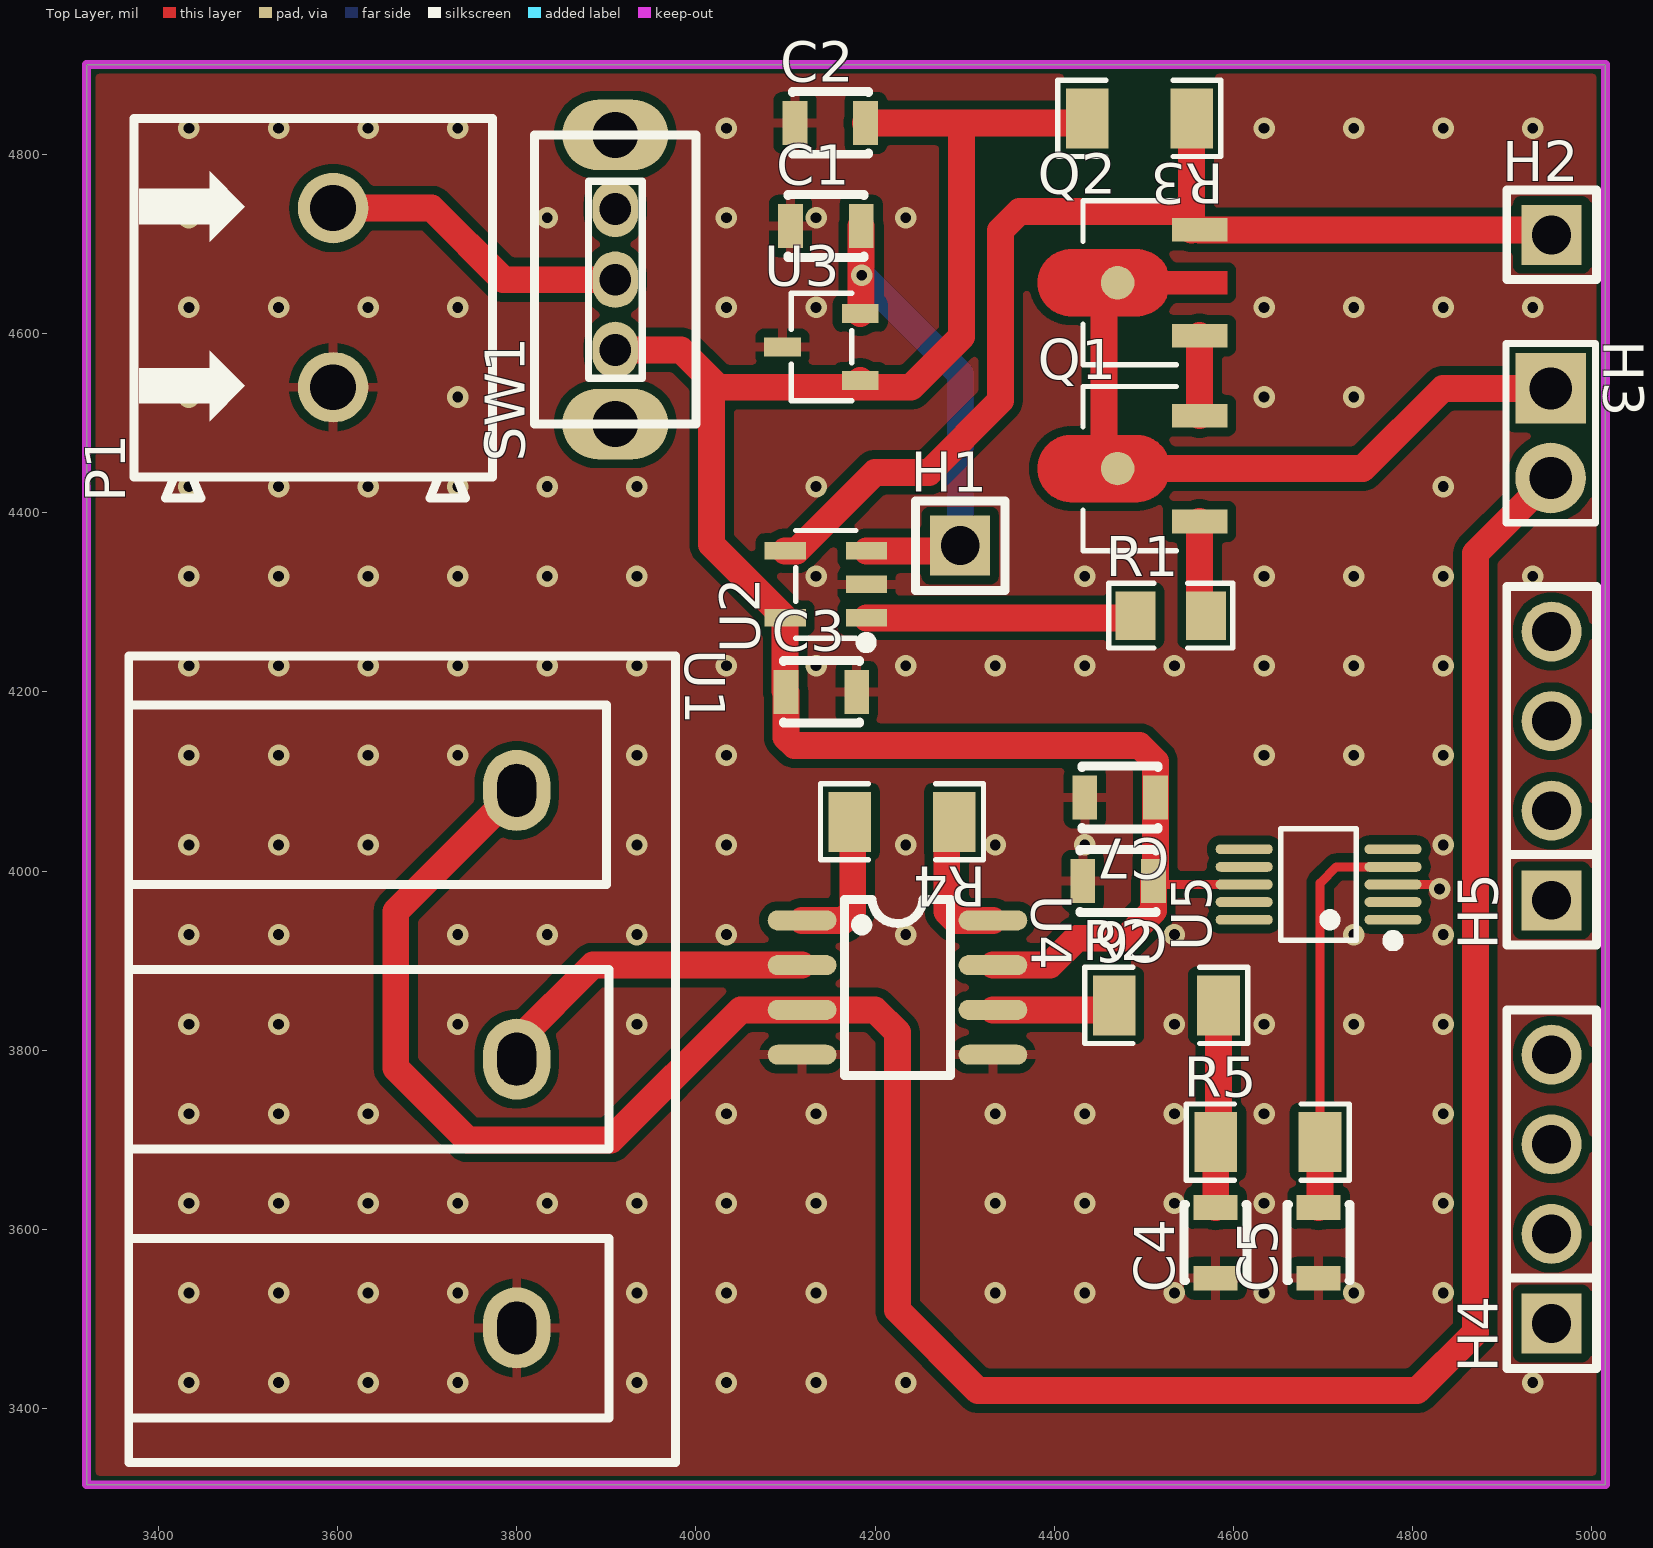
[diagram p0: Top Layer view]
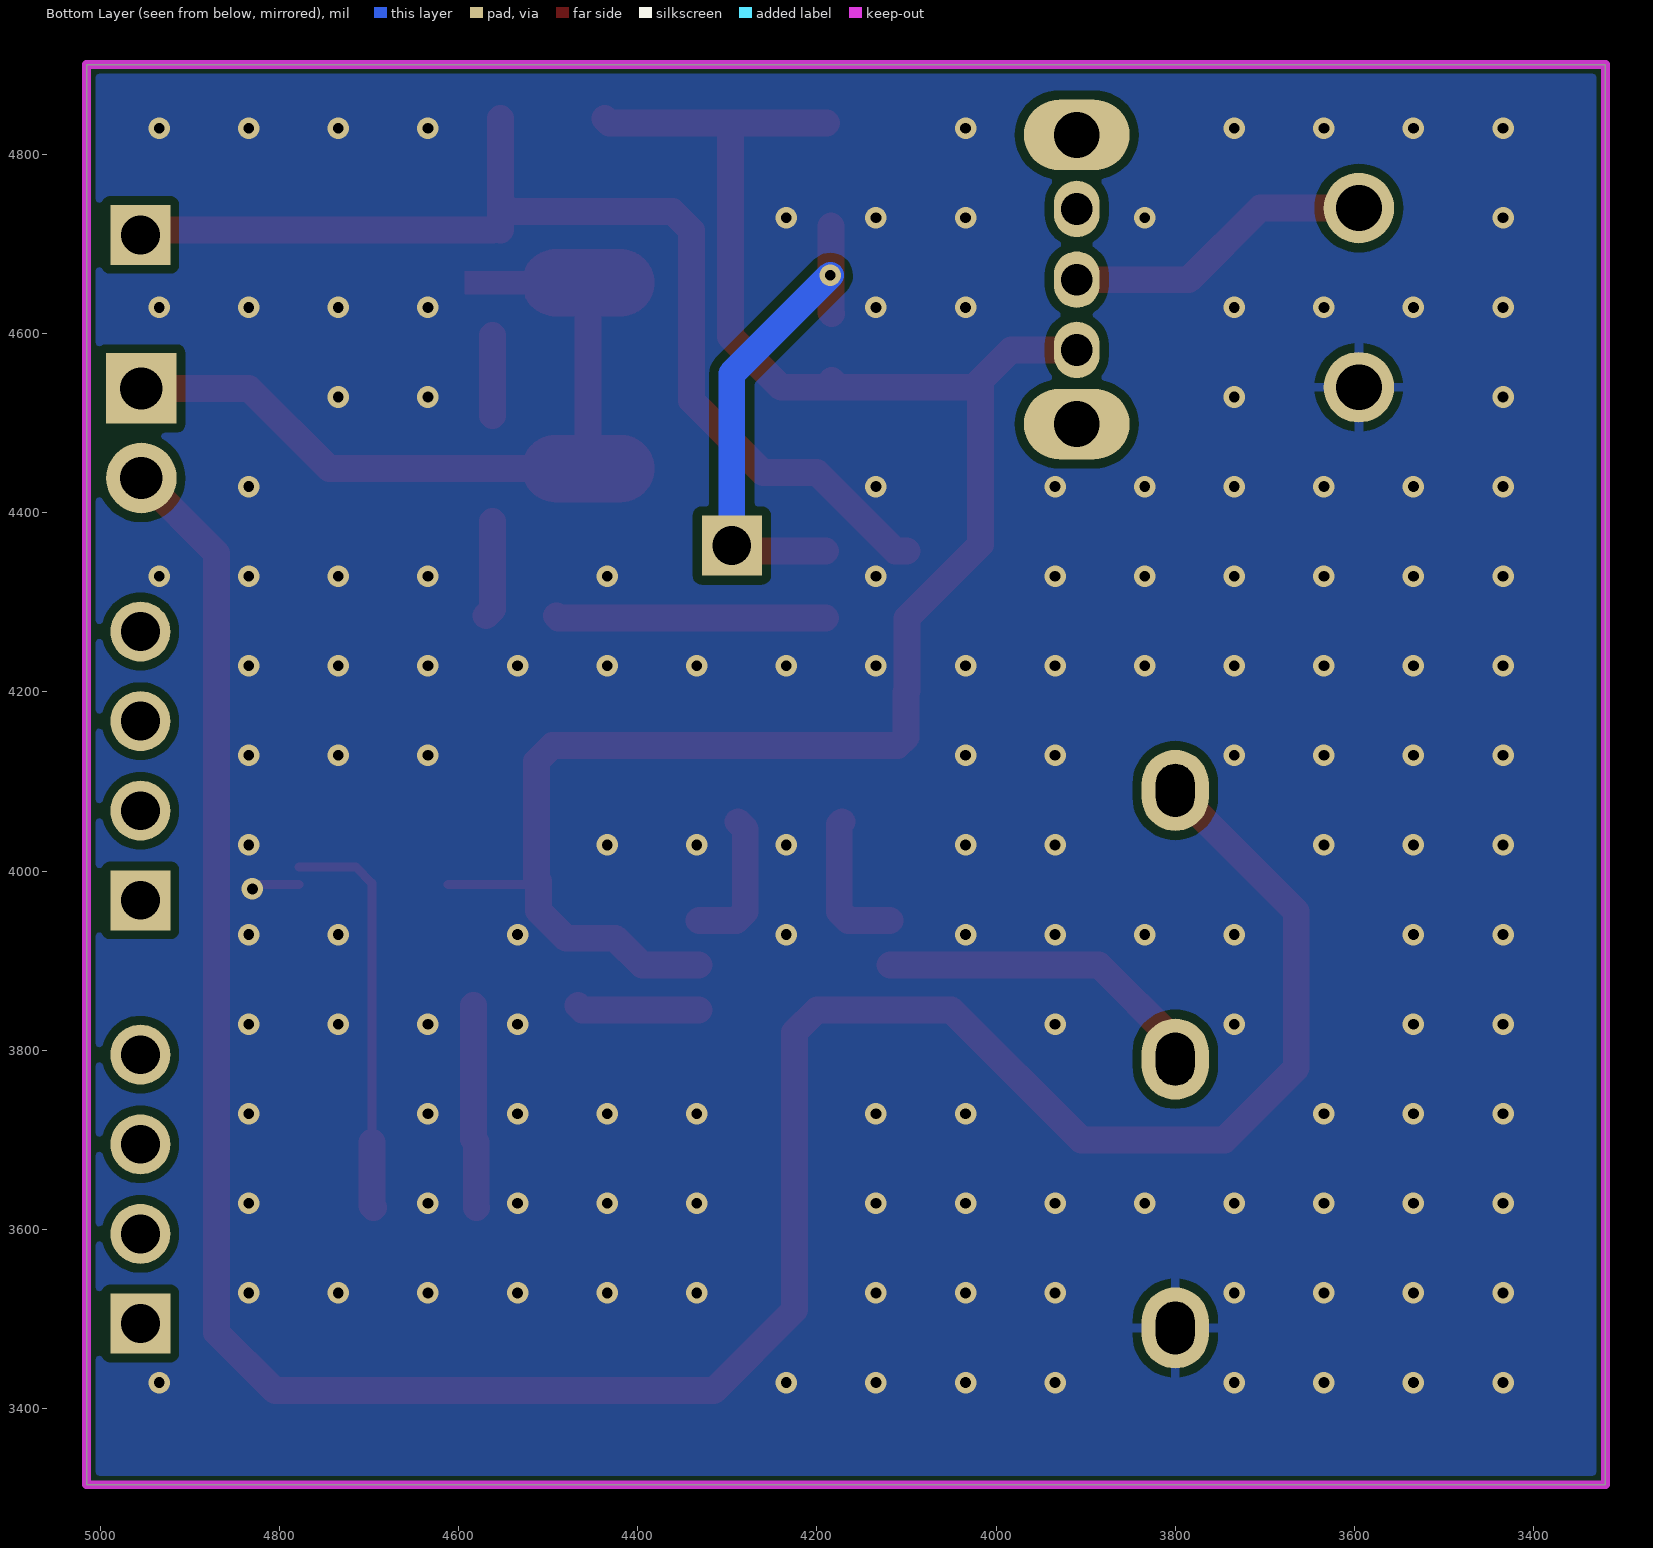
[diagram p1: Bottom Layer view, seen from below]
# Altium PCB MISC52115.pcbdoc
Units mil, origin at the board's own origin, x right, y up, seen from the top; angles counter-clockwise.
Board outline 1695 x 1585 mil, 2 copper layers (Top Layer, Bottom Layer), stack 62.206 mil thick; 26 components, 24 nets, 78 pads, 146 vias.

## Layer stack, top to bottom
Top Solder Mask Layer: solder mask 0.394, Dk 3.3
Top Layer: signal copper 1.379
Dielectric1: surface 59.449, FR4, Dk 4.5
Bottom Layer: signal copper 1.378
Bottom Solder Mask Layer: solder mask 0.394, Dk 3.3

## Board outline
3320,4900 3320,3315 5015,3315 5015,4900

## Design rules (kind name [scope] priority, off if disabled: settings)
BoardOutlineClearance copperThickness2oz_1 [All] p2 off: genericclearance=7.99 ignorepadtopadclearanceinfootprint=FALSE except(0: Arc-SplitContinuation Track-SplitContinuation SMDPad-SplitContinuation THPad-SplitContinuation Via-SplitContinuation Fill-SplitContinuation Region-SplitContinuation Poly-SplitContinuation Text-SplitContinuation Hole-SplitContinuation; 5.98: Arc-CutoutEdge SMDPad-CutoutEdge THPad-CutoutEdge Via-CutoutEdge Fill-CutoutEdge Region-CutoutEdge Text-CutoutEdge; 6.93: Hole-OutlineEdge Hole-CutoutEdge; 10: Poly-OutlineEdge Poly-CutoutEdge; 11.81: Arc-OutlineEdge Track-OutlineEdge SMDPad-OutlineEdge THPad-OutlineEdge Via-OutlineEdge Fill-OutlineEdge Region-OutlineEdge Text-OutlineEdge Track-CutoutEdge)
BoardOutlineClearance copperThickness1oz_1 [All] p4: genericclearance=4.02 ignorepadtopadclearanceinfootprint=FALSE except(0: Arc-SplitContinuation Track-SplitContinuation SMDPad-SplitContinuation THPad-SplitContinuation Via-SplitContinuation Fill-SplitContinuation Region-SplitContinuation Poly-SplitContinuation Text-SplitContinuation Hole-SplitContinuation; 6: SMDPad-CutoutEdge THPad-CutoutEdge Via-CutoutEdge Fill-CutoutEdge Region-CutoutEdge Text-CutoutEdge; 6.93: Hole-OutlineEdge Hole-CutoutEdge; 10: Poly-OutlineEdge Poly-CutoutEdge; 11.8: Arc-OutlineEdge Track-OutlineEdge SMDPad-OutlineEdge THPad-OutlineEdge Via-OutlineEdge Fill-OutlineEdge Region-OutlineEdge Text-OutlineEdge; 11.81: Arc-CutoutEdge Track-CutoutEdge)
Clearance copperThickness2oz [All] p1 off: gap=7.99 ignorepadtopadclearanceinfootprint=FALSE except(5.98: SMDPad-Track SMDPad-SMDPad THPad-Track SMDPad-THPad THPad-THPad Track-Via SMDPad-Via THPad-Via Via-Via Fill-Track Region-Track Fill-SMDPad Region-SMDPad Fill-THPad Region-THPad Fill-Via Region-Via Fill-Fill Fill-Region Region-Region Arc-Track Arc-SMDPad Arc-THPad Arc-Via Fill-Arc Region-Arc Arc-Arc Text-Track SMDPad-Text Text-THPad Text-Via Fill-Text Region-Text Arc-Text Text-Text; 6.93: Hole-Track Hole-SMDPad Hole-THPad Hole-Via Fill-Hole Region-Hole Hole-Arc Hole-Text; 10: Poly-Track Poly-SMDPad Poly-THPad Poly-Via Poly-Fill Poly-Region Poly-Poly Poly-Arc Poly-Text Poly-Hole)
Clearance copperThickness1oz [All] p3: gap=4.02 ignorepadtopadclearanceinfootprint=FALSE except(5.98: SMDPad-Track SMDPad-SMDPad THPad-Track SMDPad-THPad THPad-THPad Track-Via SMDPad-Via THPad-Via Via-Via Fill-Track Region-Track Fill-SMDPad Region-SMDPad Fill-THPad Region-THPad Fill-Via Region-Via Fill-Fill Fill-Region Region-Region; 6: Arc-Track Arc-SMDPad Arc-THPad Arc-Via Fill-Arc Region-Arc Arc-Arc Text-Track SMDPad-Text Text-THPad Text-Via Fill-Text Region-Text Arc-Text Text-Text; 6.93: Hole-Track Hole-SMDPad Hole-THPad Hole-Via Fill-Hole Region-Hole Hole-Arc Hole-Text; 10: Poly-Track Poly-SMDPad Poly-THPad Poly-Via Poly-Fill Poly-Region Poly-Poly Poly-Arc Poly-Text Poly-Hole)
DiffPairsRouting differentialPair [All] p1: maxlimit=6 minlimit=6 mostfreqgap=6 toplayer_minwidth=5 toplayer_prefwidth=10 toplayer_maxwidth=100 toplayer_mingap=6 toplayer_prefgap=6 toplayer_maxgap=6 bottomlayer_minwidth=5 bottomlayer_prefwidth=10 bottomlayer_maxwidth=100 bottomlayer_mingap=6 bottomlayer_prefgap=6 bottomlayer_maxgap=6 maxuncoupledlength=10
HoleToHoleClearance otherClearance [All] p1: gap=11.81 allowstackedmicrovias=TRUE
Length netLength [All] p1: minlimit=0 maxlimit=0
MatchedLengths netLengthTolerance [All] p1: tolerance=1000
PasteMaskExpansion pasteMaskExpansion [All] p1: expansion=0
PlaneConnect innerPlane [All] p1: planeconnectstyle=Relief reliefexpansion=20 reliefentries=4 reliefconductorwidth=10 reliefairgap=10
PolygonConnect copperRegion [(InNet('GND'))] p1: connectstyle=Relief reliefconductorwidth=10 reliefentries=4 polygonreliefangle="90 Angle" airgapwidth=10 via.connectstyle=Relief via.reliefconductorwidth=10 via.reliefentries=4 via.polygonreliefangle="90 Angle" via.airgapwidth=10
RoutingVias viaSize [All] p1: holewidth=12.01 width=24.02 viastyle="Through Hole" minholewidth=11.81 minwidth=19.68 maxholewidth=248.03 maxwidth=393.7
SolderMaskExpansion solderMaskExpansion [IsVia] p1: expansion=-1000 istentingtop=TRUE
SolderMaskExpansion solderMaskExpansion [All] p2: expansion=2 istentingtop=FALSE
Width copperThickness2oz_2 [All] p1 off: maxlimit=100 minlimit=8 preferedwidth=10
Width copperThickness1oz_2 [All] p2: maxlimit=100 minlimit=5 preferedwidth=10

## Components (designator, comment, footprint, x,y, rotation, side; value= is the part's Value field where it differs from the comment)
C1 "100nF" CAP-SMD_L2.0-W1.25 4145,4720 r0 top
C2 "100nF" CAP-SMD_L2.0-W1.25 4150,4835 r0 top
C3 "100nF" CAP-SMD_L2.0-W1.25 4140,4200 r0 top
C4 "1uF" CAP-SMD_L2.0-W1.25 4580,3585 r90 top
C5 "4.7nf" CAP-SMD_L2.0-W1.25 4695,3585 r90 top
C6 "100nf" CAP-SMD_L2.0-W1.25 4471.28,3988.83 r180 top
C7 "100nf" CAP-SMD_L2.0-W1.25 4473.49,4082.08 r180 top
H1 "PZ254V-11-01P" HDR-TH_1P-P2.54-V-M 4294.96,4363.25 r0 top
H2 "PZ254V-11-01P" HDR-TH_1P-P2.54-V-M 4955,4710 r0 top
H3 "PZ254V-11-02P" HDR-TH_2P-P2.54-V-M 4954,4488.67 r270 top
H4 "PZ254V-11-04P" HDR-TH_4P-P2.54-V-M 4955,3645 r90 top
H5 "PZ254V-11-04P" HDR-TH_4P-P2.54-V-M 4955,4117.33 r90 top
P1 "WJ500V-5.08-2P" CONN-TH_2P-P5.00_WJ500V-5.08-2P 3595,4640 r90 top
Q1 "2SA1201" SOT-89-3_L4.5-W2.5-P1.50-LS4.2-BR 4508.73,4449.26 r0 top
Q2 "2SA1201" SOT-89-3_L4.5-W2.5-P1.50-LS4.2-BR 4508.73,4656.61 r0 top
R1 "10kΩ" R0805 4530,4285 r0 top
R2 "1KΩ" R1206 4525,3850 r0 top
R3 "2.7KΩ" R1206 4495,4840 r180 top
R4 "6KΩ" R1206 4230,4055 r180 top
R5 "1KΩ" R1206 4638.39,3697.51 r0 top
SW1 "" 拨动开关 3910,4655 r90 top
U1 "JL762-76203BA1" CONN-TH_JL762-76203BA1 3800,3790 r270 top
U2 "SGM8551XN5G/TR" SOT-23-5_L3.0-W1.7-P0.95-LS2.8-BL 4145,4320 r90 top
U3 "REF3025AIDBZT" SOT-23-3_L3.0-W1.7-P0.95-LS2.9-BR 4140,4585 r0 top
U4 "AD623ARZ-R7" SOIC-8_L5.0-W4.0-P1.27-LS6.0-BL 4225,3870 r270 top
U5 "GD30AD3344" MSOP-10_L3.0-W3.0-P0.50-LS5.0-BL 4695,3985 r90 top

## Footprints (in the part's own frame and the unit in brackets; to place one, negate y for a bottom-side part, rotate by r counter-clockwise, add the part's x,y. Pads: shape width x height; smd on the part's side, far side on the other; paste and mask are expansions set on the pad)
CAP-SMD_L2.0-W1.25 [mm]
  rect 0.7x1.25 smd: 1(-1,0) 2(1,0)
  silkscreen extent -1.08,-0.89 1.08,0.89
CONN-TH_2P-P5.00_WJ500V-5.08-2P [mm]
  round 2 hole 1.3: 1(-2.54,0) 2(2.54,0)
  silkscreen extent -5.68,-4.52 5.08,5.64
CONN-TH_JL762-76203BA1 [mm]
  oval 2.3x1.9 hole 1.1 slot 1.5 at 0 deg: 1(-7.62,0) 2(0,0) 3(7.62,0)
  silkscreen extent -11.43,-11 11.43,4.5
HDR-TH_1P-P2.54-V-M [mm]
  rect 1.7x1.7 hole 1.1: 1(0,0)
  silkscreen extent -1.27,-1.27 1.27,1.27
HDR-TH_2P-P2.54-V-M [mm]
  rect 2x2 hole 1.2: 1(-1.27,0)
  round 2 hole 1.2: 2(1.27,0)
  silkscreen extent -2.54,-1.27 2.54,1.27
HDR-TH_4P-P2.54-V-M [mm]
  rect 1.7x1.7 hole 1.1: 1(-3.81,0)
  round 1.7 hole 1.1: 2(-1.27,0) 3(1.27,0) 4(3.81,0)
  silkscreen extent -5.08,-1.27 5.08,1.27
MSOP-10_L3.0-W3.0-P0.50-LS5.0-BL [mm]
  oval 0.28x1.62 smd: 1(-1,-2.11) 2(-0.5,-2.11) 3(0,-2.11) 4(0.5,-2.11) 5(1,-2.11) 6(1,2.11) 7(0.5,2.11) 8(0,2.11) 9(-0.5,2.11) 10(-1,2.11)
  silkscreen extent -1.74,-2.26 1.58,1.07
R0805 [mm]
  rect 1.133x1.377 smd paste-100 mask+0.051: 1(-1,0) 2(1,0)
  silkscreen extent -1.76,-0.92 1.76,0.92
R1206 [mil]
  rect 47.54x66.97 smd paste-3937.01 mask+2: 1(-58.22,0) 2(58.22,0)
  silkscreen extent -91,-42 91,42
SOIC-8_L5.0-W4.0-P1.27-LS6.0-BL [mil]
  oval 22.38x76.78 smd: 1(-75,-106.5) 2(-25,-106.5) 3(25,-106.5) 4(75,-106.5) 5(75,106.5) 6(25,106.5) 7(-25,106.5) 8(-75,106.5)
  silkscreen extent -98,-59 98,59
SOT-23-3_L3.0-W1.7-P0.95-LS2.9-BR [mil]
  rect 40.85x20.95 smd: 1(43.36,-37.4) 2(43.36,37.4) 3(-43.36,0)
  silkscreen extent -34,-60 34,60
SOT-23-5_L3.0-W1.7-P0.95-LS2.8-BL [mm]
  rect 0.49x1.157 smd: 1(-0.95,-1.154) 2(0,-1.154) 3(0.95,-1.154)
  rect 0.49x1.175 smd: 4(0.95,1.154) 5(-0.95,1.154)
  silkscreen extent -1.8,-1.29 1.53,0.85
SOT-89-3_L4.5-W2.5-P1.50-LS4.2-BR [mm]
  rect 1.575x0.672 smd: 1(1.356,-1.5) 3(1.356,1.5)
  round 0.95 smd: 2(-0.966,0)
  Top Layer region: -2.283,0.95 -0.429,0.95 -0.384,0.949 -0.34,0.946 -0.296,0.94 -0.252,0.933 -0.208,0.924 -0.165,0.912 -0.123,0.899 -0.081,0.884 -0.04,0.866 0,0.847 0.04,0.826 0.078,0.803 0.115,0.779 0.151,0.752 0.185,0.724 0.219,0.695 0.251,0.664 0.281,0.631 0.31,0.597 0.337,0.562 0.362,0.525 0.386,0.488 0.408,0.449 0.428,0.409 0.447,0.33 2.144,0.33 2.144,-0.33 0.447,-0.33 0.428,-0.409 0.408,-0.449 0.386,-0.488 0.362,-0.526 0.337,-0.562 0.31,-0.597 0.281,-0.631 0.251,-0.664 0.219,-0.695 0.185,-0.725 0.151,-0.753 0.115,-0.779 0.078,-0.804 0.04,-0.827 0,-0.848 -0.04,-0.867 -0.081,-0.884 -0.123,-0.899 -0.165,-0.913 -0.208,-0.924 -0.252,-0.934 -0.296,-0.941 -0.34,-0.946 -0.384,-0.949 -0.429,-0.95 -2.283,-0.95 -2.328,-0.949 -2.372,-0.946 -2.416,-0.941 -2.46,-0.934 -2.504,-0.924 -2.547,-0.913 -2.589,-0.899 -2.631,-0.884 -2.672,-0.867 -2.713,-0.848 -2.752,-0.827 -2.79,-0.804 -2.827,-0.779 -2.863,-0.753 -2.898,-0.725 -2.931,-0.695 -2.963,-0.664 -2.993,-0.631 -3.022,-0.597 -3.049,-0.562 -3.075,-0.526 -3.098,-0.488 -3.12,-0.449 -3.141,-0.409 -3.159,-0.369 -3.175,-0.327 -3.189,-0.285 -3.202,-0.242 -3.212,-0.199 -3.22,-0.155 -3.227,-0.111 -3.231,-0.067 -3.233,-0.022 -3.233,0.022 -3.231,0.067 -3.227,0.111 -3.22,0.155 -3.212,0.199 -3.202,0.242 -3.189,0.285 -3.175,0.327 -3.159,0.369 -3.141,0.409 -3.12,0.449 -3.098,0.488 -3.075,0.525 -3.049,0.562 -3.022,0.597 -2.993,0.631 -2.963,0.664 -2.931,0.695 -2.898,0.724 -2.863,0.752 -2.827,0.779 -2.79,0.803 -2.752,0.826 -2.713,0.847 -2.672,0.866 -2.631,0.884 -2.589,0.899 -2.547,0.912 -2.504,0.924 -2.46,0.933 -2.416,0.94 -2.372,0.946 -2.328,0.949
  silkscreen extent -1.95,-2.33 0.7,2.33
拨动开关 [mil]
  oval 63x51.2 hole 35.4 paste+0 mask+2: 1(-73.4,0) 2(5,0) 3(84,0)
  oval 78.7x118.1 hole 51.2 paste+0 mask+2: 4(166.7,0) 5(-156.1,0)
  silkscreen extent -156,-90 167,90

## Via types
v1: diameter 24.02, hole 12, Top Layer to Bottom Layer, 146 vias

## Nets (pads, with @x,y where several pads share a name; then routed paths per layer and width w, separated by ;. In a path a pad name is that pad's centre, name@x,y a point inside that pad or via, vN(x,y) a via of type N, cw(c..) or ccw(c..) an arc to the next point about the centre after c; other vN are vias at no path point)
$1N4: C1.2 H1.1 U2.3 U3.2 | length 552.3
  Top Layer w30: U3.2 4184.37,4623.41 C1.2 ; U2.3 4289.11,4357.4 H1.1
  Bottom Layer w30: v1(4185,4665) 4294.96,4555.04 H1.1
$1N8: R1.1 U2.1 | length 301.2
  Top Layer w30: U2.1 4488.23,4282.6 R1.1
$1N10: Q1.1 R1.2 | length 108.2
  Top Layer w30: Q1.1 4562.13,4292.24 R1.2
$1N11: Q1.3 Q2.1 | length 89.2
  Top Layer w30: Q1.3 Q2.1
$1N12: H2.1 Q2.3 R3.1 U2.4 | length 1245.8
  Top Layer w30: U2.4 4112.4,4357.4 4200,4445 4260,4445 4340,4525 4340,4715 4361.21,4736.21 4542.56,4736.21 4553.22,4746.87 ; Q2.3@4553.22,4715.67 4553.22,4746.87 ; R3.1 4553.22,4746.87 ; Q2.3 4949.33,4715.67 H2.1
$1N18: H3.1 Q1.2 Q2.2 | length 743.1
  Top Layer w30: Q2.2@4455.34,4656.61 4455.34,4449.25 4744.25,4449.25 4833.67,4538.67 H3.1
$1N34: R4.2 U4.1 | length 162
  Top Layer w30: U4.1 4165,3945 4175,3955 4175,4051.78 R4.2
$1N35: U1.2 U4.2 | length 373.7
  Top Layer w30: U1.2 3800,3810 3885,3895 U4.2
$1N36: R4.1 U4.8 | length 159
  Top Layer w30: R4.1 4280,4046.78 4280,3955 4290,3945 U4.8
$1N40: R2.1 U4.6 | length 137.4
  Top Layer w30: U4.6 4461.78,3845 R2.1
$1N41: C4.2 R2.2 R5.1 | length 227
  Top Layer w30: C4.2 4580.17,3624.54 R5.1 4583.22,3700.57 R2.2
$1N43: C5.2 R5.2 U5.4 | length 451.9
  Top Layer w10: R5.2 4696.61,3986.61 4714.69,4004.69 U5.4
  Top Layer w30: C5.2 4696.61,3625.98 R5.2
$1N48: H4.1
$1N49: H4.2
$1N50: H4.3
$1N51: H4.4
$1N52: H5.1
$1N53: H5.2
$1N54: H5.3
$1N55: H5.4
$1N62: P1.2 SW1.2 | length 348.1
  Top Layer w30: P1.2 3705,4740 3785,4660 SW1.2
+5V: C2.2 C3.1 C6.1 C7.1 R3.2 SW1.1 U2.5 U3.1 U4.7 U5.8 | length 2256.4
  Top Layer w10: C6.1 4514.48,3985 U5.8
  Top Layer w30: SW1.1 3983.4,4581.6 4017.56,4547.44 ; U3.1 U3.1@4175.76,4540 ; C2.2 4296.39,4835 ; U4.7 4395,3895 4425,3925 4480,3925 4510.65,3955.65 C6.1 4512.86,3991.04 C7.1 4512.86,4122.14 4495,4140 4110,4140 4100.63,4149.37 C3.1 4099.58,4201.05 U2.5 4017.56,4364.62 4017.56,4547.44 ; R3.2 4431.78,4835 4296.39,4835 ; 4017.56,4547.44 4025,4540 U3.1@4175.76,4540 ; U3.1@4175.76,4540 4240,4540 4296.39,4596.39 4296.39,4835
GND: C1.1 C2.1 C3.2 C4.1 C5.1 C6.2 C7.2 P1.1 U1.3 U2.2 U3.3 U4.4 U4.5 U5.3 | length 54
  Top Layer w10: U5.3 4825,3985 v1(4830,3980)
  other v1: 3434.1,3429.1 3534.1,3429.1 3634.1,3429.1 3734.1,3429.1 3934.1,3429.1 4034.1,3429.1 4134.1,3429.1 4234.1,3429.1 4934.1,3429.1 3434.1,3529.1 3534.1,3529.1 3634.1,3529.1 3734.1,3529.1 3934.1,3529.1 4034.1,3529.1 4134.1,3529.1 4334.1,3529.1 4434.1,3529.1 4534.1,3529.1 4634.1,3529.1 4734.1,3529.1 4834.1,3529.1 3434.1,3629.1 3534.1,3629.1 3634.1,3629.1 3734.1,3629.1 3834.1,3629.1 3934.1,3629.1 4034.1,3629.1 4134.1,3629.1 4334.1,3629.1 4434.1,3629.1 4534.1,3629.1 4634.1,3629.1 4834.1,3629.1 3434.1,3729.1 3534.1,3729.1 3634.1,3729.1 4034.1,3729.1 4134.1,3729.1 4334.1,3729.1 4434.1,3729.1 4534.1,3729.1 4634.1,3729.1 4834.1,3729.1 3434.1,3829.1 3534.1,3829.1 3734.1,3829.1 3934.1,3829.1 4534.1,3829.1 4634.1,3829.1 4734.1,3829.1 4834.1,3829.1 3434.1,3929.1 3534.1,3929.1 3734.1,3929.1 3834.1,3929.1 3934.1,3929.1 4034.1,3929.1 4234.1,3929.1 4534.1,3929.1 4734.1,3929.1 4834.1,3929.1 3434.1,4029.1 3534.1,4029.1 3634.1,4029.1 3934.1,4029.1 4034.1,4029.1 4234.1,4029.1 4334.1,4029.1 4434.1,4029.1 4834.1,4029.1 3434.1,4129.1 3534.1,4129.1 3634.1,4129.1 3734.1,4129.1 3934.1,4129.1 4034.1,4129.1 4634.1,4129.1 4734.1,4129.1 4834.1,4129.1 3434.1,4229.1 3534.1,4229.1 3634.1,4229.1 3734.1,4229.1 3834.1,4229.1 3934.1,4229.1 4034.1,4229.1 4134.1,4229.1 4234.1,4229.1 4334.1,4229.1 4434.1,4229.1 4534.1,4229.1 4634.1,4229.1 4734.1,4229.1 4834.1,4229.1 3434.1,4329.1 3534.1,4329.1 3634.1,4329.1 3734.1,4329.1 3834.1,4329.1 3934.1,4329.1 4134.1,4329.1 4434.1,4329.1 4634.1,4329.1 4734.1,4329.1 4834.1,4329.1 4934.1,4329.1 3434.1,4429.1 3534.1,4429.1 3634.1,4429.1 3734.1,4429.1 3834.1,4429.1 3934.1,4429.1 4134.1,4429.1 4834.1,4429.1 3434.1,4529.1 3734.1,4529.1 4634.1,4529.1 4734.1,4529.1 3434.1,4629.1 3534.1,4629.1 3634.1,4629.1 3734.1,4629.1 4034.1,4629.1 4134.1,4629.1 4634.1,4629.1 4734.1,4629.1 4834.1,4629.1 4934.1,4629.1 3434.1,4729.1 3834.1,4729.1 4034.1,4729.1 4134.1,4729.1 4234.1,4729.1 3434.1,4829.1 3534.1,4829.1 3634.1,4829.1 3734.1,4829.1 4034.1,4829.1 4634.1,4829.1 4734.1,4829.1 4834.1,4829.1 4934.1,4829.1
PT100: H3.2 U1.1 U4.3 | length 3037.1
  Top Layer w30: U1.1 3665,3955 3665,3780 3745,3700 3905,3700 4050,3845 U4.3 4200,3845 4225,3820 4225,3510 4315,3420 4805,3420 4870,3485 4870,4354.67 H3.2
pads on no net: SW1.3 SW1.4 SW1.5 U5.1 U5.2 U5.5 U5.6 U5.7 U5.9 U5.10

## Polygon pours and split planes (outlines as drawn)
GND on Top Layer (solid, remove dead copper, pour order 0): 3105,4915 3105,3000 5510,3000 5510,4915
GND on Bottom Layer (solid, remove dead copper, pour order 2): 3000,5080 3000,3015 5385,3015 5385,5080

## Keep-outs
Board Outline Layer:
  the board outline again, w10